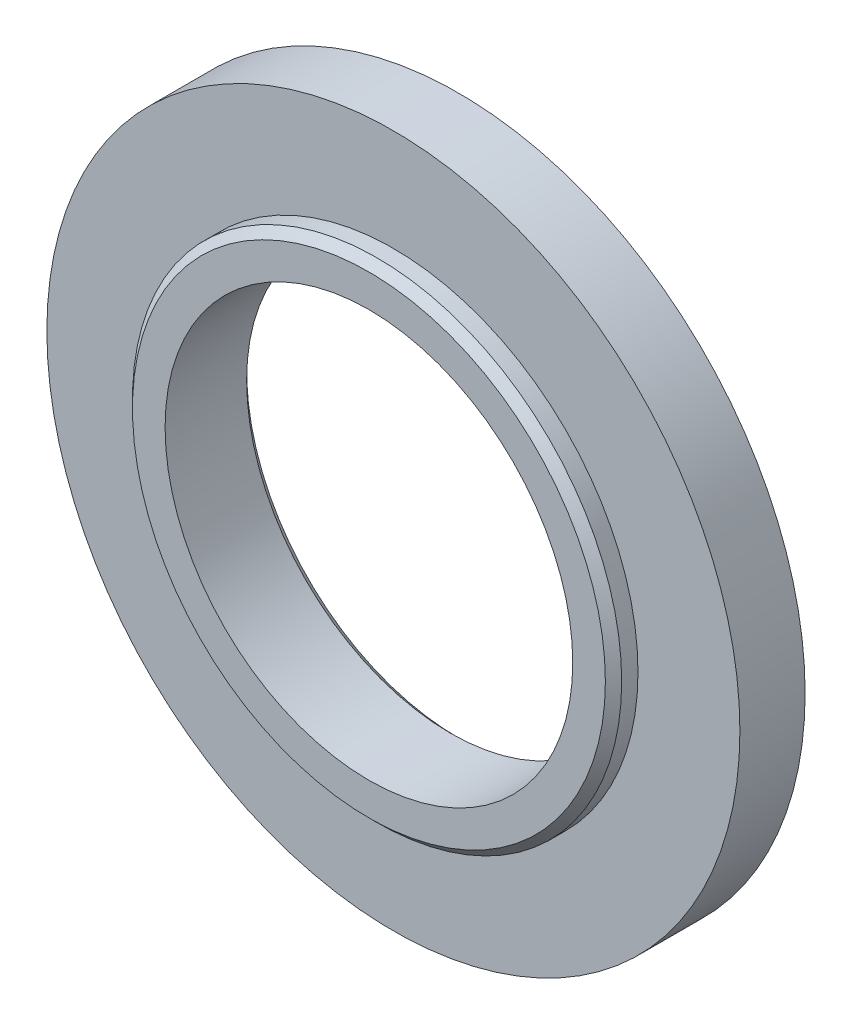
SolidWorks part; units mm, degrees
ref_plane "Front Plane" through (0, 0, 0) normal (0, 0, 1) x (1, 0, 0)
ref_plane "Top Plane" through (0, 0, 0) normal (0, 1, 0) x (1, 0, 0)
ref_plane "Right Plane" through (0, 0, 0) normal (1, 0, 0) x (0, 0, -1)
sketch "Sketch1" plane through (0, 0, 0) normal (0, 0, 1) x (1, 0, 0)
  circle A0 centre (0, 0) radius 42.5
  circle A1 centre (0, 0) radius 25
extrude "Boss-Extrude1" add sketch "Sketch1" along normal blind 8
sketch "Sketch2" plane through (0, 0, 8) normal (0, 0, 1) x (1, 0, 0)
  circle A0 centre (0, 0) radius 30
  circle A1 centre (0, 0) radius 25
extrude "Boss-Extrude2" add sketch "Sketch2" along normal blind 3
chamfer "Chamfer1" distance 1 distance2 1 2 edges at (25, 0, 0) (30, 0, 11)
sketch "Sketch3" plane through (0, 0, 0) normal (0, 0, -1) x (-1, 0, 0)
  circle A0 centre (0, 0) radius 37 construction
  circle A1 centre (37, 0) radius 1.925
  circle A2 centre (18.5, -32.0429) radius 1.925
  circle A3 centre (-18.5, -32.0429) radius 1.925
  circle A4 centre (-37, 0) radius 1.925
  circle A5 centre (-18.5, 32.0429) radius 1.925
  circle A6 centre (18.5, 32.0429) radius 1.925
  point P17 (0, 0)
  dimension "D1" = 6
hole_wizard "M4 Tapped Hole1" positions "3DSketch1" profile "Sketch4" tap size "M4" standard "Gb"
sketch3d "3DSketch1"
  point P0 (18.5, 32.0429, 0)
  point P3 (-18.5, 32.0429, 0)
  point P6 (-37, 0, 0)
  point P9 (-18.5, -32.0429, 0)
  point P12 (18.5, -32.0429, 0)
  point P15 (37, 0, 0)
sketch "Sketch4" plane through (18.5, 32.0429, 0) normal (1, 0, 0) x (0, 1, 0)
  line L0 (0, 0) -> (0, 6.9914)
  line L1 (0, 6.9914) -> (1.65, 6)
  line L2 (1.65, 6) -> (1.65, 0)
  line L5 (1.65, 0) -> (0, 0)
  line L10 (0, 6.9914) -> (-1.65, 6) construction
  line L11 (0, -6.35) -> (0, 107.95) construction
  dimension "螺纹孔钻头直径" = 3.3
  dimension "螺纹孔钻头深度" = 6
  dimension "导头角度" = 118
cosmetic thread "Hole Thread1" parameters "D1"=5, "D2"=4
cosmetic thread "Hole Thread2" parameters "D1"=5, "D2"=4
cosmetic thread "Hole Thread3" parameters "D1"=5, "D2"=4
cosmetic thread "Hole Thread4" parameters "D1"=5, "D2"=4
cosmetic thread "Hole Thread5" parameters "D1"=5, "D2"=4
cosmetic thread "Hole Thread6" parameters "D1"=5, "D2"=4
